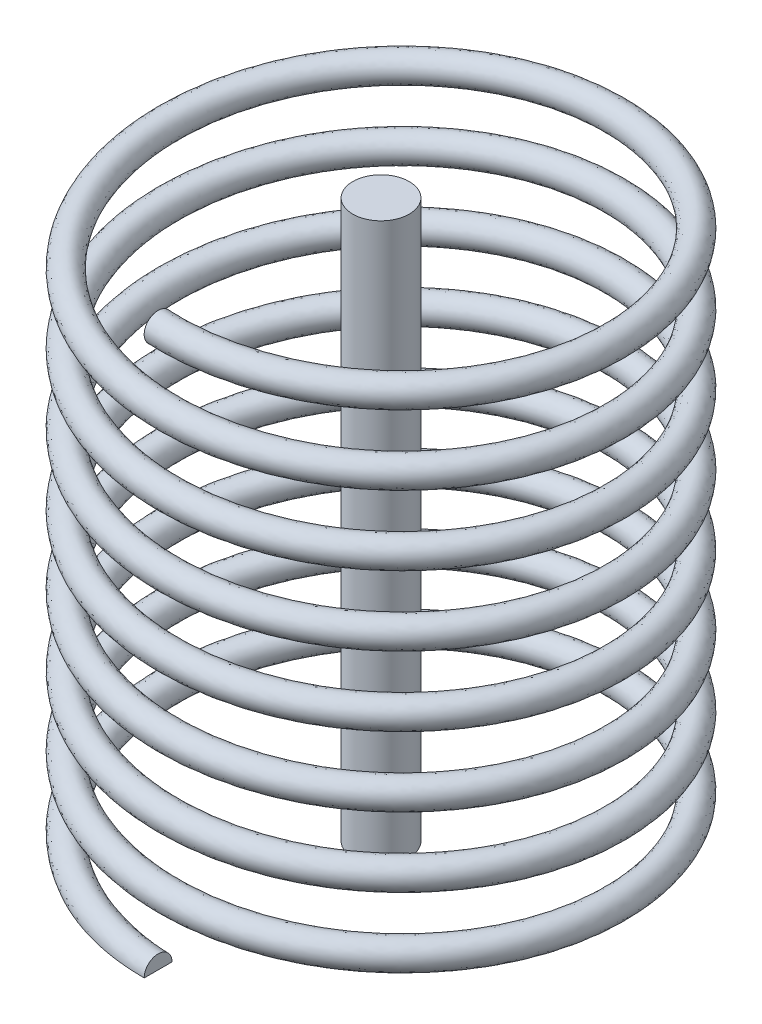
from build123d import *

# Parameters (mm, degrees)
SWEEP_1_PITCH       = 1.25
SWEEP_1_HEIGHT      = 10
SWEEP_1_RADIUS      = 4
SKETCH_3_R          = 0.25
SKETCH_4_R          = 5.626020109
CUT_EXTRUDE_1_DEPTH = 10
SKETCH_5_R          = 0.506602862
EXTRUDE_1_DEPTH     = 10


with BuildPart() as part:
    # 扫描1: sweep along a helix
    with BuildLine() as sweep_1_path:
        Helix(SWEEP_1_PITCH, SWEEP_1_HEIGHT, SWEEP_1_RADIUS, center=(0, 0, 0), direction=(0, 1, 0), lefthand=True)
    # 草图3 → 扫描1 (sweep)
    with BuildSketch(Plane(origin=(0, 0, 0), x_dir=(0, 0, -1), z_dir=(1, 0, 0))):
        with Locations((-4, 0)):
            Circle(SKETCH_3_R)
    sweep(path=sweep_1_path.line, is_frenet=True)

    # 草图4 → 切除-拉伸1 (cut)
    with BuildSketch(Plane(origin=(0, 0, 0), x_dir=(1, 0, 0), z_dir=(0, 1, 0))):
        Circle(SKETCH_4_R)
    extrude(amount=-CUT_EXTRUDE_1_DEPTH, mode=Mode.SUBTRACT)


with BuildPart() as body_2:
    # 草图5 → 凸台-拉伸1 (new body)
    with BuildSketch(Plane.XZ):
        with Locations(Location((0, 0, 0), (0, 0, 270))):
            Circle(SKETCH_5_R)
    extrude(amount=-EXTRUDE_1_DEPTH)


solid = Compound([part.part, body_2.part])
